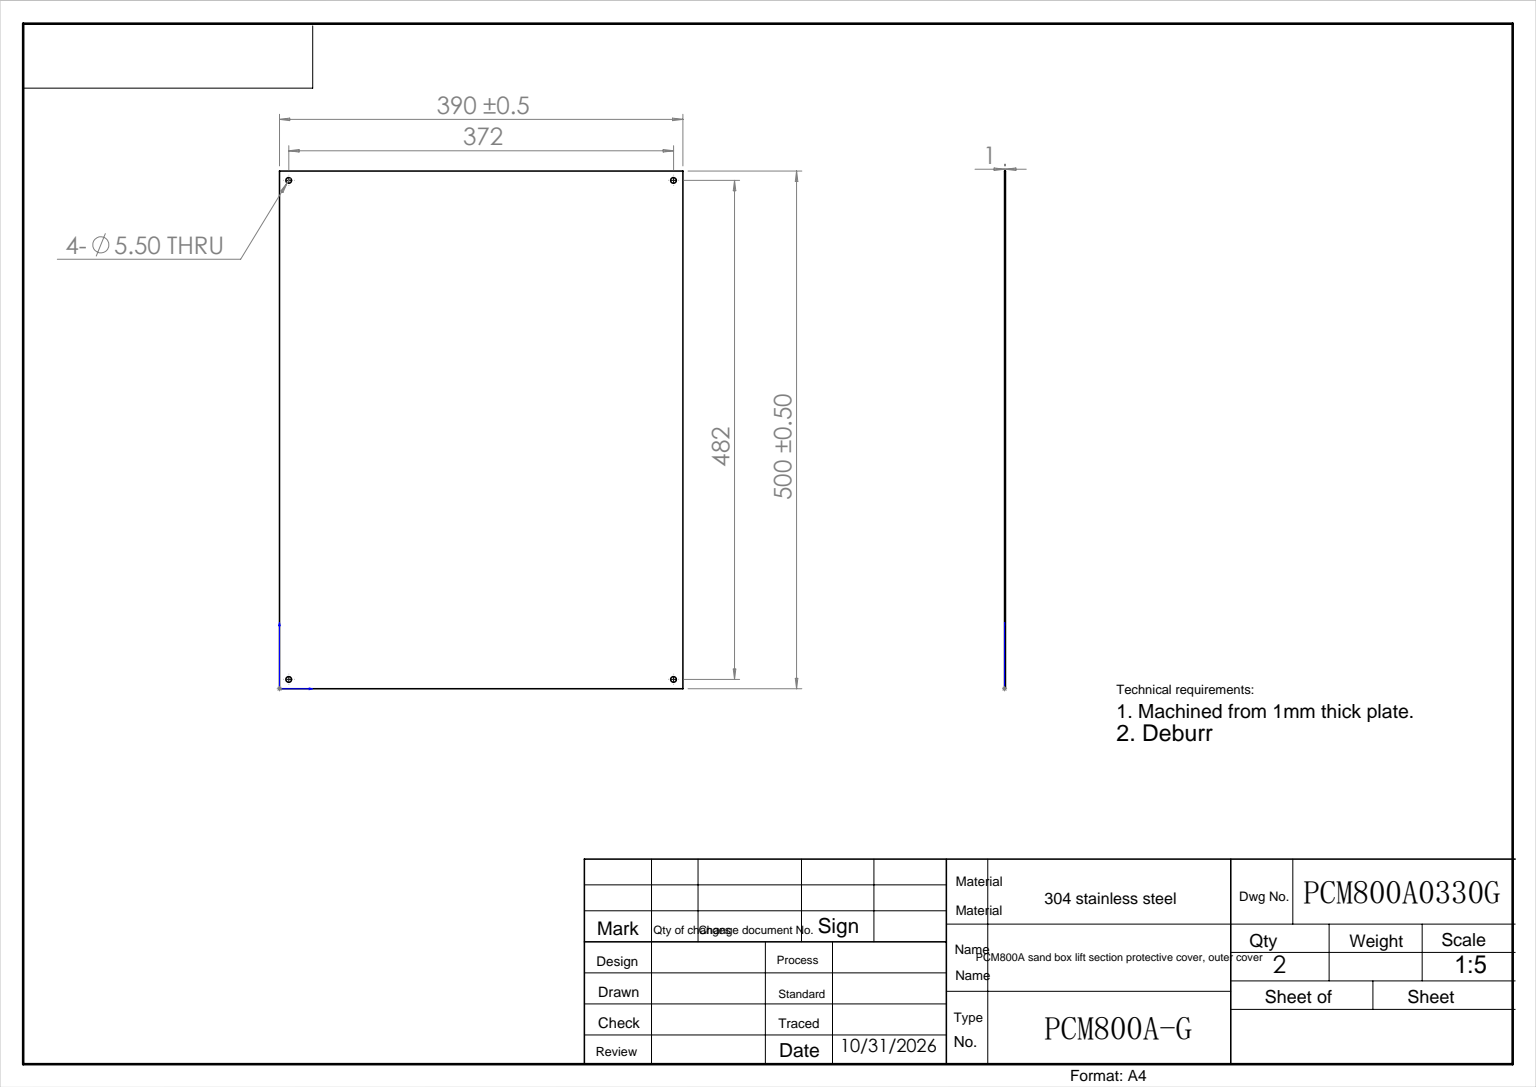
from build123d import *

# Parameters (mm, degrees)
SKETCH_1_W          = 390
SKETCH_1_H          = 500
EXTRUDE_1_DEPTH     = 1
SKETCH_2_R          = 2.75
CUT_EXTRUDE_1_DEPTH = 1


with BuildPart() as part:
    # 草图1 → 凸台-拉伸1 (new body)
    with BuildSketch(Plane.XY):
        with Locations((195, 250)):
            Rectangle(SKETCH_1_W, SKETCH_1_H)
    extrude(amount=EXTRUDE_1_DEPTH)

    # 草图2 → 切除-拉伸1 (cut)
    with BuildSketch(Plane.XY.offset(1)):
        with Locations((9, 491)):
            Circle(SKETCH_2_R)
        with Locations((381, 491)):
            Circle(SKETCH_2_R)
        with Locations((9, 9)):
            Circle(SKETCH_2_R)
        with Locations((381, 9)):
            Circle(SKETCH_2_R)
    extrude(amount=-CUT_EXTRUDE_1_DEPTH, mode=Mode.SUBTRACT)


solid = part.part
